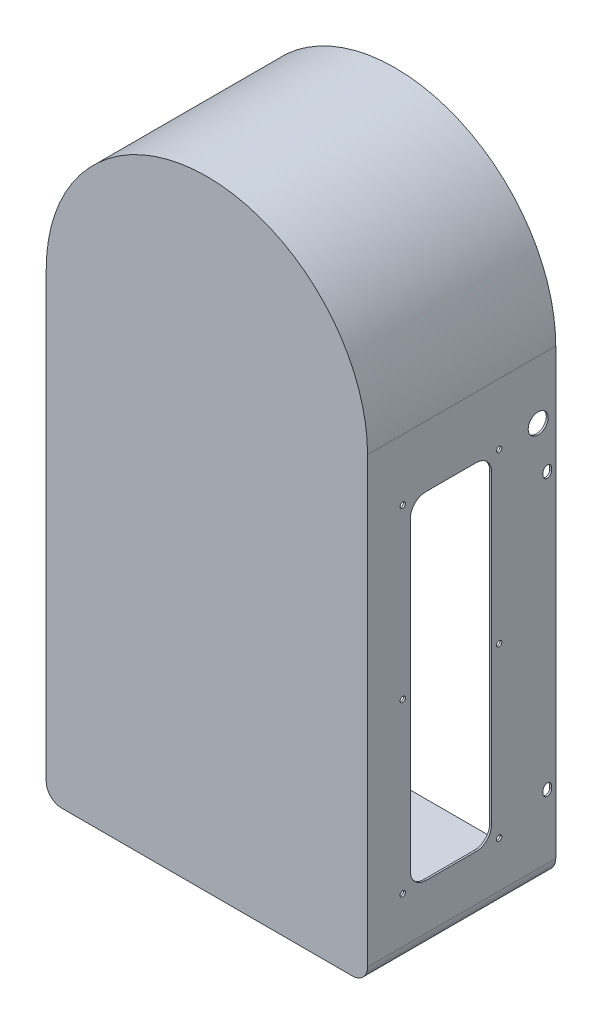
SolidWorks part; units mm, degrees
material "普通碳钢"
ref_plane "Front Plane" through (0, 0, 0) normal (0, 0, 1) x (1, 0, 0)
ref_plane "Top Plane" through (0, 0, 0) normal (0, 1, 0) x (1, 0, 0)
ref_plane "Right Plane" through (0, 0, 0) normal (1, 0, 0) x (0, 0, -1)
sketch "Sketch1" plane through (0, 0, 0) normal (0, 0, 1) x (1, 0, 0)
  line L0 (-105, -150.6) -> (-105, 149.4)
  line L1 (93.8, -149.4) -> (-93.8, -149.4)
  line L2 (103.8, -139.4) -> (103.8, 149.4)
  line L4 (-103.8, -139.4) -> (-103.8, 149.4)
  line L5 (103.8, -149.4) -> (-103.8, 149.4) construction
  line L6 (103.8, 149.4) -> (-103.8, -149.4) construction
  line L7 (105, -150.6) -> (-105, -150.6)
  line L8 (105, -150.6) -> (105, 149.4)
  line L9 (103.8, -149.4) -> (-103.8, -149.4) construction
  line L10 (103.8, -149.4) -> (103.8, 149.4) construction
  line L11 (-103.8, -149.4) -> (-103.8, 149.4) construction
  arc A0 (103.8, 149.4) -> (-103.8, 149.4) centre (0, 149.4) ccw
  arc A1 (105, 149.4) -> (-105, 149.4) centre (0, 149.4) ccw
  arc A2 (93.8, -149.4) -> (103.8, -139.4) centre (93.8, -139.4) ccw
  arc A3 (-103.8, -139.4) -> (-93.8, -149.4) centre (-93.8, -139.4) ccw
  point P0 (0, 0)
  dimension "D3" = 1.2
  dimension "D4" = 10
  dimension "D1" = 207.6
  dimension "D2" = 298.8
extrude "Boss-Extrude1" add sketch "Sketch1" along normal blind 123
sketch "Sketch2" plane through (0, 0, 123) normal (0, 0, 1) x (1, 0, 0)
  line L3 (-105, 149.4) -> (-105, -150.6)
  line L4 (-105, -150.6) -> (105, -150.6)
  line L5 (105, -150.6) -> (105, 149.4)
  line L6 (-105, 149.4) -> (-105, -150.6)
  line L7 (-105, -150.6) -> (105, -150.6)
  line L8 (105, -150.6) -> (105, 149.4)
  arc A1 (105, 149.4) -> (-105, 149.4) centre (0, 149.4) ccw
  arc A2 (105, 149.4) -> (-105, 149.4) centre (0, 149.4) ccw
  dimension "D1" = 0
extrude "Boss-Extrude2" add sketch "Sketch2" against normal blind 1.2
fillet "Fillet1" radius 10 1 edges at (-105, -150.6, 61.5)
fillet "Fillet2" radius 10 1 edges at (105, -150.6, 61.5)
sketch "Sketch3" plane through (-105, 0, 0) normal (-1, 0, 0) x (0, 0, 1)
  line L0 (5.5, 80.1) -> (5.5, 82.1) construction
  line L1 (2.75, 80.1) -> (2.75, 82.1)
  line L2 (8.25, 80.1) -> (8.25, 82.1)
  line L3 (5.5, -99.9) -> (5.5, -97.9) construction
  line L4 (2.75, -99.9) -> (2.75, -97.9)
  line L5 (8.25, -99.9) -> (8.25, -97.9)
  line L6 (0, 149.4) -> (0, -140.6) construction
  line L7 (123, -150.6) -> (0, -150.6) construction
  arc A0 (2.75, 80.1) -> (8.25, 80.1) centre (5.5, 80.1) ccw
  arc A1 (8.25, 82.1) -> (2.75, 82.1) centre (5.5, 82.1) ccw
  arc A2 (2.75, -99.9) -> (8.25, -99.9) centre (5.5, -99.9) ccw
  arc A3 (8.25, -97.9) -> (2.75, -97.9) centre (5.5, -97.9) ccw
  point P2 (5.5, 81.1)
  point P8 (5.5, -98.9)
  dimension "D2" = 2.75
  dimension "D1" = 2
  dimension "D3" = 5.5
  dimension "D4" = 51.7
  dimension "D5" = 180
extrude "Cut-Extrude1" cut sketch "Sketch3" against normal through all
sketch "Sketch4" plane through (-105, 0, 0) normal (-1, 0, 0) x (0, 0, 1)
  line L5 (123, -150.6) -> (0, -150.6) construction
  line L6 (0, 149.4) -> (0, -140.6) construction
  line L12 (123, 149.4) -> (0, 149.4) construction
  circle A0 centre (1.5, -48.6) radius 6 construction
  circle A2 centre (11.5, 111.4) radius 6.5
  dimension "D1" = 12
  dimension "D2" = 102
  dimension "D3" = 1.5
  dimension "D4" = 11.5
  dimension "D5" = 13
  dimension "D6" = 38
extrude "Cut-Extrude2" cut sketch "Sketch4" against normal through all
sketch "Sketch5" plane through (105, 0, 0) normal (1, 0, 0) x (0, 0, -1)
  line L0 (-95, 109.4) -> (-95, -110.6)
  line L1 (-95, 109.4) -> (-42, 109.4)
  line L2 (-95, -110.6) -> (-42, -110.6)
  line L3 (-42, 109.4) -> (-42, -110.6)
  line L4 (0, -140.6) -> (0, 149.4) construction
  line L6 (-123, -140.6) -> (-123, 149.4) construction
  line L8 (-76.9343, -0.6) -> (40.8415, -0.6) construction
  line L11 (-123, 149.4) -> (0, 149.4) construction
  dimension "D1" = 42
  dimension "D2" = 150
  dimension "D3" = 28
  dimension "D4" = 220
extrude "Cut-Extrude3" cut sketch "Sketch5" against normal through all
fillet "Fillet3" radius 10 8 edges at (-104.4, 109.4, 42) (-104.4, 109.4, 95) (-104.4, -110.6, 95) (-104.4, -110.6, 42) (104.4, -110.6, 42) (104.4, -110.6, 95) (104.4, 109.4, 95) (104.4, 109.4, 42)
sketch "Sketch6" plane through (105, 0, 0) normal (1, 0, 0) x (0, 0, -1)
  line L0 (-42, -0.6) -> (30.7422, -0.6) construction
  line L1 (-42, -100.6) -> (-42, 99.4) construction
  line L2 (-68.5, 109.4) -> (-68.5, -125.376) construction
  line L3 (-52, 109.4) -> (-85, 109.4) construction
  circle A0 centre (-37, 109.4) radius 1.75
  circle A1 centre (-37, -0.6) radius 1.75
  circle A2 centre (-37, -110.6) radius 1.75
  circle A3 centre (-100, -110.6) radius 1.75
  circle A4 centre (-100, -0.6) radius 1.75
  circle A5 centre (-100, 109.4) radius 1.75
  dimension "D1" = 3.5
  dimension "D3" = 5
  dimension "D2" = 220
extrude "Cut-Extrude4" cut sketch "Sketch6" against normal through all
